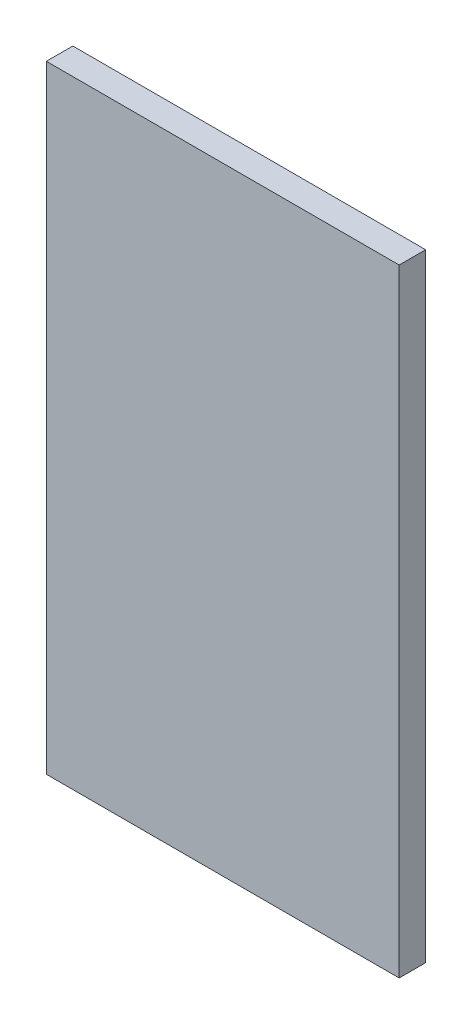
SolidWorks part; units mm, degrees
ref_plane "前视基准面" through (0, 0, 0) normal (0, 0, 1) x (1, 0, 0)
ref_plane "上视基准面" through (0, 0, 0) normal (0, 1, 0) x (1, 0, 0)
ref_plane "右视基准面" through (0, 0, 0) normal (1, 0, 0) x (0, 0, -1)
sketch "草图1" plane through (0, 0, 0) normal (0, 0, 1) x (1, 0, 0)
  line L0 (0, 0) -> (40, 0)
  line L1 (40, 0) -> (40, 70)
  line L2 (40, 70) -> (0, 70)
  line L3 (0, 70) -> (0, 0)
extrude "凸台-拉伸1" add sketch "草图1" along normal blind 3
